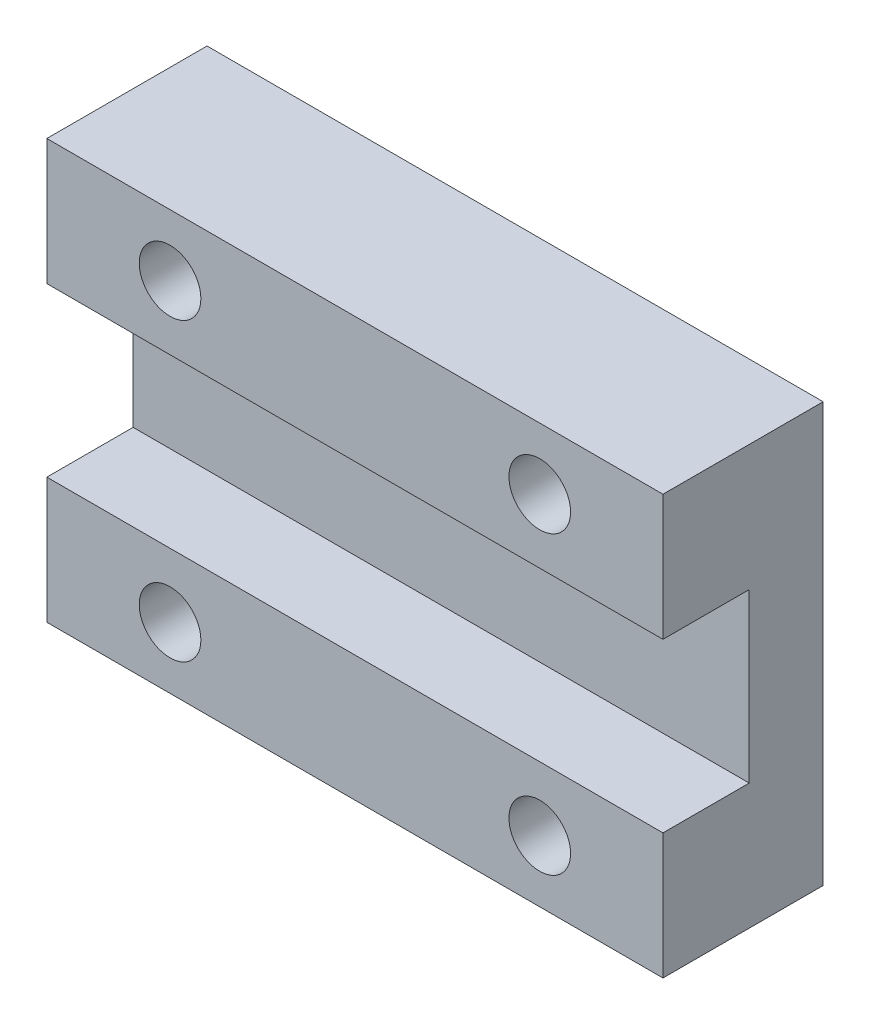
from build123d import *

# Parameters (mm, degrees)
SKETCH_1_W          = 25
SKETCH_1_H          = 17
EXTRUDE_1_DEPTH     = 6.5
CUT_EXTRUDE_1_REACH = 30.286
SKETCH_2_W          = 3.5
SKETCH_2_H          = 6.8
CUT_EXTRUDE_2_REACH = 20.562
SKETCH_3_R          = 1.25


with BuildPart() as part:
    # 草图1 → 凸台-拉伸1 (new body)
    with BuildSketch(Plane.XY):
        with Locations((-0.517429194, 3.026143791)):
            Rectangle(SKETCH_1_W, SKETCH_1_H)
    extrude(amount=EXTRUDE_1_DEPTH)

    # 草图2 → 切除-拉伸1 (cut, up to next)
    with BuildSketch(Plane(origin=(11.982570806, 0, 0), x_dir=(0, 0, -1), z_dir=(1, 0, 0)), mode=Mode.PRIVATE) as cut_extrude_1_sk1:
        with Locations((-4.75, 3.026143791)):
            Rectangle(SKETCH_2_W, SKETCH_2_H)
    cut_extrude_1_tool1 = extrude(cut_extrude_1_sk1.sketch, amount=-CUT_EXTRUDE_1_REACH, mode=Mode.PRIVATE) & part.part
    add(cut_extrude_1_tool1.solids().sort_by_distance((11.982571, 3.026144, 4.75))[0], mode=Mode.SUBTRACT)

    # 草图3 → 切除-拉伸2 (cut, up to next)
    with BuildSketch(Plane.XY.offset(6.5), mode=Mode.PRIVATE) as cut_extrude_2_sk1:
        with Locations((-8.017429194, 9.026143791)):
            Circle(SKETCH_3_R)
    cut_extrude_2_tool1 = extrude(cut_extrude_2_sk1.sketch, amount=-CUT_EXTRUDE_2_REACH, mode=Mode.PRIVATE) & part.part
    # 草图3 → 切除-拉伸2 (cut, up to next)
    with BuildSketch(Plane.XY.offset(6.5), mode=Mode.PRIVATE) as cut_extrude_2_sk2:
        with Locations((6.982570806, 9.026143791)):
            Circle(SKETCH_3_R)
    cut_extrude_2_tool2 = extrude(cut_extrude_2_sk2.sketch, amount=-CUT_EXTRUDE_2_REACH, mode=Mode.PRIVATE) & part.part
    # 草图3 → 切除-拉伸2 (cut, up to next)
    with BuildSketch(Plane.XY.offset(6.5), mode=Mode.PRIVATE) as cut_extrude_2_sk3:
        with Locations((-8.017429194, -2.973856209)):
            Circle(SKETCH_3_R)
    cut_extrude_2_tool3 = extrude(cut_extrude_2_sk3.sketch, amount=-CUT_EXTRUDE_2_REACH, mode=Mode.PRIVATE) & part.part
    # 草图3 → 切除-拉伸2 (cut, up to next)
    with BuildSketch(Plane.XY.offset(6.5), mode=Mode.PRIVATE) as cut_extrude_2_sk4:
        with Locations((6.982570806, -2.973856209)):
            Circle(SKETCH_3_R)
    cut_extrude_2_tool4 = extrude(cut_extrude_2_sk4.sketch, amount=-CUT_EXTRUDE_2_REACH, mode=Mode.PRIVATE) & part.part
    add(cut_extrude_2_tool1.solids().sort_by_distance((-8.017429, 9.026144, 6.5))[0], mode=Mode.SUBTRACT)
    add(cut_extrude_2_tool2.solids().sort_by_distance((6.982571, 9.026144, 6.5))[0], mode=Mode.SUBTRACT)
    add(cut_extrude_2_tool3.solids().sort_by_distance((-8.017429, -2.973856, 6.5))[0], mode=Mode.SUBTRACT)
    add(cut_extrude_2_tool4.solids().sort_by_distance((6.982571, -2.973856, 6.5))[0], mode=Mode.SUBTRACT)


solid = part.part
